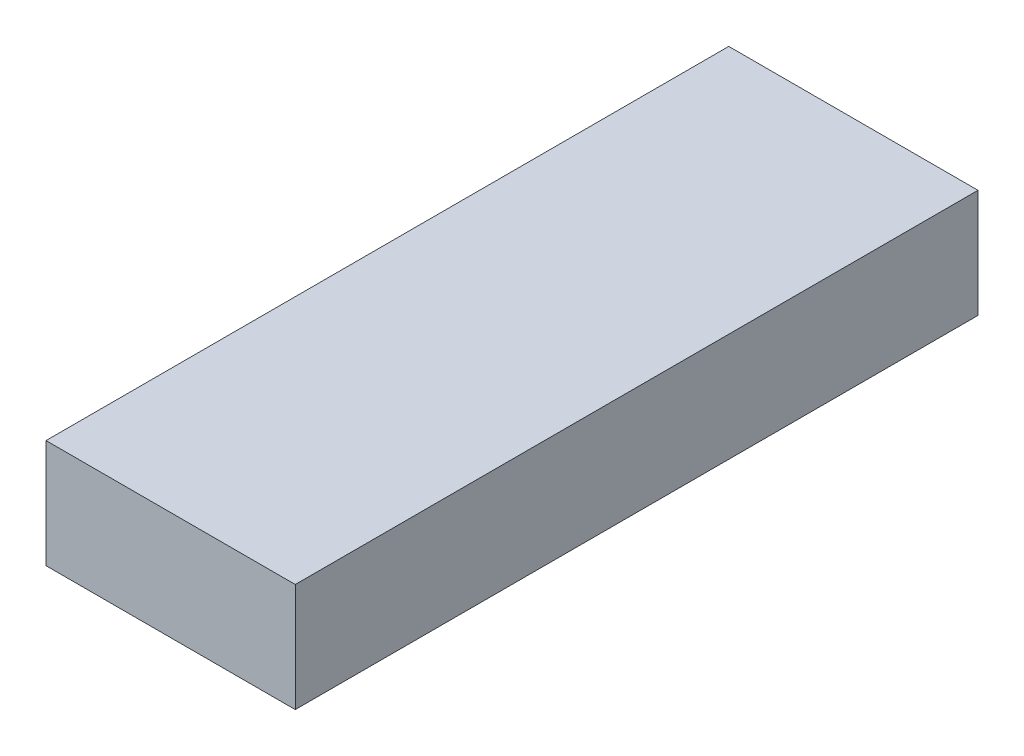
SolidWorks part; units mm, degrees
material "Q235"
ref_plane "前视基准面" through (0, 0, 0) normal (0, 0, 1) x (1, 0, 0)
ref_plane "上视基准面" through (0, 0, 0) normal (0, 1, 0) x (1, 0, 0)
ref_plane "右视基准面" through (0, 0, 0) normal (1, 0, 0) x (0, 0, -1)
sketch "草图1" plane through (0, 0, 0) normal (0, 1, 0) x (1, 0, 0)
  line L1 (0, 0) -> (23, 0)
  line L2 (0, 0) -> (0, 63)
  line L3 (0, 63) -> (23, 63)
  line L4 (23, 0) -> (23, 63)
  dimension "D1" = 63
  dimension "D2" = 23
extrude "凸台-拉伸1" add sketch "草图1" along normal blind 10
